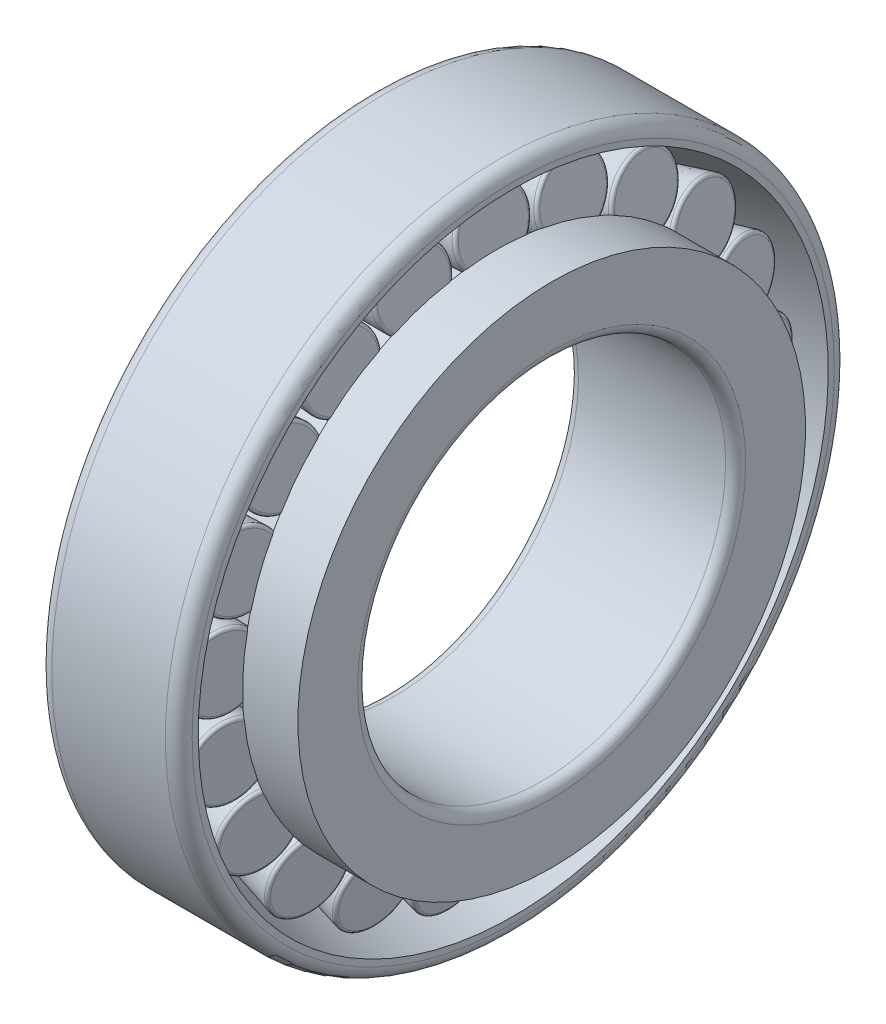
SolidWorks part; units mm, degrees
ref_plane "Front" through (0, 0, 0) normal (0, 0, 1) x (1, 0, 0)
ref_plane "Top" through (0, 0, 0) normal (0, 1, 0) x (1, 0, 0)
ref_plane "Right" through (0, 0, 0) normal (1, 0, 0) x (0, 0, -1)
other "Configuration Table"
sketch "Sketch1" plane through (0, 0, 0) normal (0, 0, 1) x (1, 0, 0)
  line L0 (16.25, 0) -> (13.9916, 0) construction
  line L1 (10.5, 47.0883) -> (10.5, 48)
  line L2 (8.5, 50) -> (-8.5, 50)
  line L3 (-10.5, 48) -> (-10.5, 41.4185)
  line L4 (-10.5, 41.4185) -> (10.5, 47.0883)
  line L5 (-8.75, 29) -> (-8.75, 35.1542)
  line L6 (-7.25, 27.5) -> (14.75, 27.5)
  line L7 (16.25, 29) -> (16.25, 37.9398)
  line L8 (-5.8796, 33.6542) -> (-7.4125, 42.2521)
  line L9 (8.5, 34.9398) -> (6.5254, 46.0152)
  line L10 (-6.646, 37.9531) -> (7.5127, 40.4775) construction
  line L11 (-5.8796, 33.6542) -> (8.5, 34.9398)
  line L12 (7.9651, 38.75) -> (16.25, 38.75)
  line L13 (16.25, 37.9398) -> (7.9651, 37.9398)
  line L14 (-8.75, 35.1542) -> (-6.147, 35.1542)
  arc A0 (-8.5, 50) -> (-10.5, 48) centre (-8.5, 48) ccw
  arc A1 (10.5, 48) -> (8.5, 50) centre (8.5, 48) ccw
  arc A2 (-7.25, 27.5) -> (-8.75, 29) centre (-7.25, 29) cw
  arc A3 (14.75, 27.5) -> (16.25, 29) centre (14.75, 29) ccw
  point P19 (-10.5, 50)
  point P22 (10.5, 50)
  point P24 (0, 50)
  point P29 (-8.75, 27.5)
  point P32 (16.25, 27.5)
revolve "Revolve1" add sketch "Sketch1" angle 360 about L0
sketch "Sketch2" plane through (0, 0, 0) normal (0, 0, 1) x (1, 0, 0)
  line L0 (-6.6657, 37.9496) -> (6.538, 40.3037) construction
  line L4 (-6.646, 37.9531) -> (7.5127, 40.4775) construction
  line L5 (-6.6657, 37.9496) -> (7.5324, 40.481)
  line L7 (-7.4322, 42.2486) -> (-5.8961, 33.6326)
  line L8 (8.5235, 34.9218) -> (6.5451, 46.0187)
  line L9 (-5.8961, 33.6326) -> (8.5235, 34.9218)
  line L10 (-6.6657, 37.9496) -> (-5.9684, 34.0386)
  line L11 (8.4373, 35.4053) -> (7.5324, 40.481)
  line L12 (-5.4854, 33.6694) -> (8.0344, 34.8781)
  arc A0 (-5.4854, 33.6694) -> (-5.9684, 34.0386) centre (-5.5254, 34.1176) cw
  arc A1 (8.0344, 34.8781) -> (8.4373, 35.4053) centre (7.9943, 35.3263) ccw
revolve "Revolve2" add sketch "Sketch2" angle 360 about L0
sketch "Sketch3" plane through (0, 0, 0) normal (0, 0, 1) x (1, 0, 0)
  line L0 (-10.5, 41.4185) -> (10.5, 47.0883) construction
  line L1 (-10.5, 48) -> (-10.5, 41.4185) construction
  line L2 (8.5, 50) -> (-8.5, 50) construction
  line L3 (10.5, 47.0883) -> (10.5, 48) construction
  line L4 (-10.5, 41.4185) -> (10.5, 47.0883)
  line L5 (-10.5, 48) -> (-10.5, 41.4185)
  line L6 (8.5, 50) -> (-8.5, 50)
  line L7 (10.5, 47.0883) -> (10.5, 48)
  arc A0 (-8.5, 50) -> (-10.5, 48) centre (-8.5, 48) ccw construction
  arc A1 (10.5, 48) -> (8.5, 50) centre (8.5, 48) ccw construction
  arc A2 (-8.5, 50) -> (-10.5, 48) centre (-8.5, 48) ccw
  arc A3 (10.5, 48) -> (8.5, 50) centre (8.5, 48) ccw
revolve "Revolve3" add sketch "Sketch3" angle 360 about axis through (16.25, 0, 0) along (-1, 0, 0)
pattern_circular "Circular-Pattern1" count 21 over 360 about axis through (0, 0, 0) along (1, 0, 0) of "Revolve2"
equation "\"gzzj@Sketch1\" =  ( \"DD@Sketch1\" - \"XD@Sketch1\" )  / 4"
equation "\"D1@Sketch1\" = \"DB@Sketch1\" - \"DT@Sketch1\" / 20"
equation "\"D2@Sketch1\" = \"DT@Sketch1\" - \"DC@Sketch1\" + \"XR12@Sketch1\""
equation "\"D4@Sketch1\" = \"D3@Sketch1\" / 2"
equation "\"D2@Sketch2\" = \"gzzj@Sketch1\" / 25"
equation "\"ZJ@Sketch1\" =  ( \"DD@Sketch1\" + \"XD@Sketch1\" )  / 2"
equation "\"D1@Circular-Pattern1\" = int( 3.14159265 / atn(( \"gzzj@Sketch1\" / 2) / sqr( \"ZJ@Sketch1\" * \"ZJ@Sketch1\" /4 - ( \"gzzj@Sketch1\"/ 2) *  ( \"gzzj@Sketch1\"/ 2))))"
